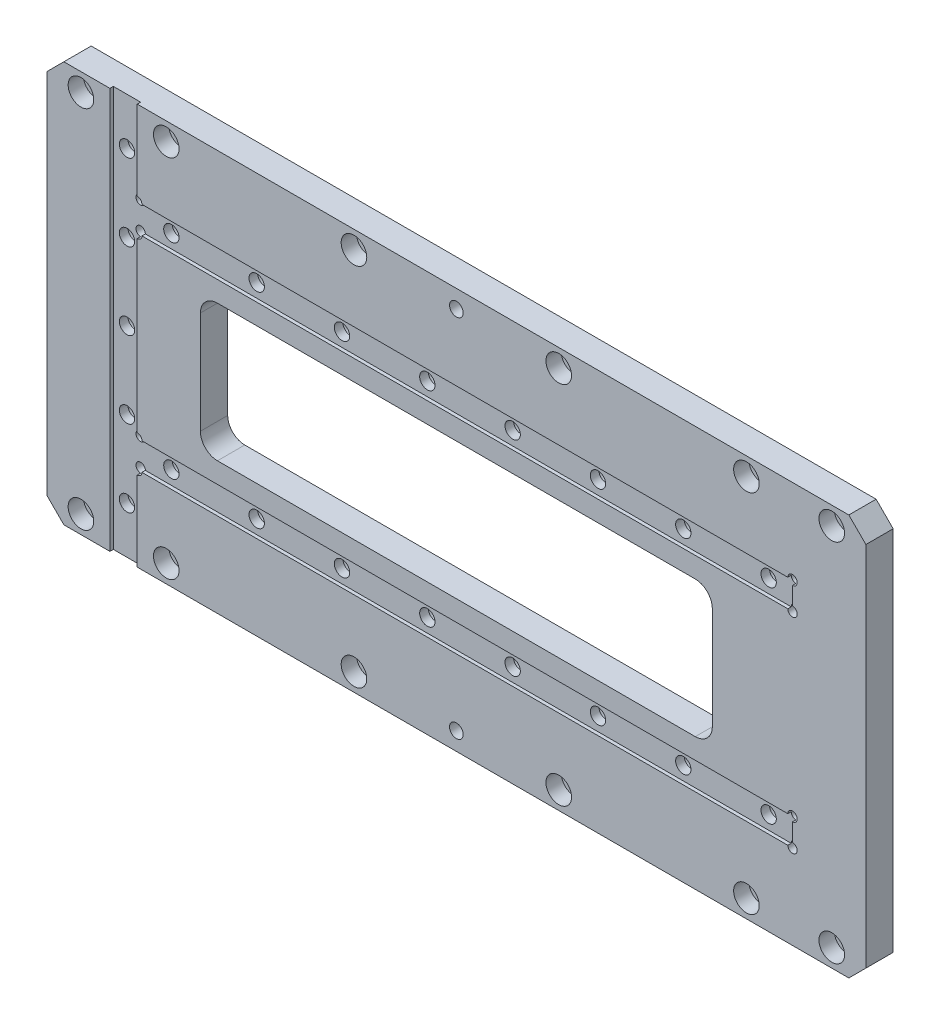
SolidWorks part; units mm, degrees
material "6061 合金"
ref_plane "Front" through (0, 0, 0) normal (0, 0, 1) x (1, 0, 0)
ref_plane "Top" through (0, 0, 0) normal (0, 1, 0) x (1, 0, 0)
ref_plane "Right" through (0, 0, 0) normal (1, 0, 0) x (0, 0, -1)
sketch "草图1" plane through (0, 0, 0) normal (0, 0, 1) x (1, 0, 0)
  line L2 (-240, -117.5) -> (-240, 117.5)
  line L3 (-240, 117.5) -> (240, 117.5)
  line L4 (240, -117.5) -> (240, 117.5)
  line L5 (-240, -117.5) -> (240, 117.5) construction
  line L6 (-240, 117.5) -> (240, -117.5) construction
  line L15 (-240, -117.5) -> (240, -117.5)
  dimension "D1" = 235
  dimension "D2" = 480
extrude "凸台-拉伸1" add sketch "草图1" along normal blind 16
hole_wizard "打孔尺寸(%根据)内六角圆柱头螺钉的类型1" positions "草图10" profile "草图11" counterbore size "M8" standard "GB" end condition through all
sketch "草图10" plane through (0, 0, 16) normal (0, 0, 1) x (1, 0, 0)
  line L8 (-220, 107) -> (220, 107) construction
  line L9 (-220, 107) -> (-220, -107) construction
  line L10 (-220, -107) -> (220, -107) construction
  line L11 (220, 107) -> (220, -107) construction
  line L12 (0, 117.5) -> (0, -117.2465) construction
  line L13 (-240, 117.5) -> (240, 117.5) construction
  line L14 (-240, 0) -> (240, 0) construction
  line L15 (-240, -117.5) -> (-240, 117.5) construction
  line L16 (240, -117.5) -> (240, 117.5) construction
  line L17 (-170, 107) -> (-170, -107) construction
  line L18 (-60, 107) -> (-60, -107) construction
  line L19 (60, 107) -> (60, -107) construction
  line L20 (170, 107) -> (170, -107) construction
  point P316 (-220, 107)
  point P317 (220, -107)
  point P420 (-220, -107)
  point P421 (220, 107)
  point P437 (-170, 107)
  point P438 (-170, -107)
  point P439 (-60, 107)
  point P440 (-60, -107)
  point P442 (60, 107)
  point P443 (60, -107)
  point P444 (170, 107)
  point P445 (170, -107)
  dimension "D1" = 214
  dimension "D2" = 440
  dimension "D3" = 120
  dimension "D4" = 340
sketch "草图11" plane through (-220, 107, 16) normal (1, 0, 0) x (0, -1, 0)
  line L0 (0, 0) -> (0, 16)
  line L1 (0, 16) -> (4.5, 16)
  line L3 (4.5, 16) -> (4.5, 9)
  line L4 (4.5, 9) -> (7.5, 9)
  line L5 (7.5, 9) -> (7.5, 0)
  line L7 (7.5, 0) -> (0, 0)
  line L11 (0, -6.35) -> (0, 107.95) construction
  dimension "通孔孔直径" = 9
  dimension "通孔孔深度" = 16
  dimension "柱形沉头孔直径" = 15
  dimension "柱形沉头孔深度" = 9
chamfer "倒角1" distance 10 angle 45 4 edges at (240, 117.5, 8) (240, -117.5, 8) (-240, -117.5, 8) (-240, 117.5, 8)
hole_wizard "大小mm 暗销孔1" positions "草图12" profile "草图13" hole size "Ø8.0" standard "GB" end condition through all
sketch "草图12" plane through (0, 0, 16) normal (0, 0, 1) x (1, 0, 0)
  line L1 (-60, 107) -> (60, 107) construction
  line L2 (-60, -107) -> (60, -107) construction
  point P12 (0, 107)
  point P14 (0, -107)
sketch "草图13" plane through (0, -107, 16) normal (1, 0, 0) x (0, -1, 0)
  line L0 (0, 0) -> (0, 16)
  line L1 (0, 16) -> (4, 16)
  line L2 (4, 16) -> (4, 0)
  line L5 (4, 0) -> (0, 0)
  line L11 (0, -6.35) -> (0, 107.95) construction
  dimension "通孔孔直径" = 8
  dimension "通孔孔深度" = 16
sketch "草图16" plane through (0, 0, 16) normal (0, 0, 1) x (1, 0, 0)
  line L0 (-240, 0) -> (240, 0) construction
  line L1 (-240, -107.5) -> (-240, 107.5) construction
  line L2 (240, -107.5) -> (240, 107.5) construction
  line L3 (-195, 117.5) -> (-195, -117.5) construction
  line L4 (-230, 117.5) -> (230, 117.5) construction
  line L5 (0, 117.5) -> (0, -117.5) construction
  line L6 (-230, -117.5) -> (230, -117.5) construction
  line L8 (-203, -117.5) -> (-187, -117.5)
  line L9 (-203, -117.5) -> (-203, 117.5)
  line L10 (-203, 117.5) -> (-187, 117.5)
  line L11 (-187, -117.5) -> (-187, 117.5)
  line L12 (-195, 117.5) -> (-195, -117.5) construction
  line L13 (-203, 0) -> (-187, 0) construction
  point P14 (-195, 0)
  dimension "D1" = 16
  dimension "D2" = 195
extrude "切除-拉伸1" cut sketch "草图16" against normal blind 2
sketch "草图17" plane through (0, 0, 16) normal (0, 0, 1) x (1, 0, 0)
  line L1 (-240, -107.5) -> (-240, 107.5) construction
  line L2 (-240, 0) -> (240, 0) construction
  line L3 (-203, 60) -> (-240, 60) construction
  line L4 (-203, 117.5) -> (-203, -117.5) construction
  line L5 (-240, -47.5) -> (-203, -47.5) construction
  line L6 (-203, -68) -> (-203, -52)
  line L7 (197, 68) -> (-203, 68)
  line L8 (197, 68) -> (197, 52)
  line L9 (197, 52) -> (-203, 52)
  line L10 (-203, 68) -> (-203, 52)
  line L11 (197, -52) -> (-203, -52)
  line L12 (197, -68) -> (197, -52)
  line L13 (197, -68) -> (-203, -68)
  line L14 (240, -107.5) -> (240, 107.5) construction
  dimension "D2" = 16
  dimension "D3" = 400
  dimension "D5" = 120
extrude "切除-拉伸2" cut sketch "草图17" against normal blind 2
sketch "草图18" plane through (0, 0, 16) normal (0, 0, 1) x (1, 0, 0)
  line L0 (-187, 52) -> (197, 52) construction
  line L1 (-150, -40) -> (150, -40)
  line L2 (-150, -40) -> (-150, 40)
  line L3 (-150, 40) -> (150, 40)
  line L4 (150, -40) -> (150, 40)
  line L5 (0, 40) -> (0, -40) construction
  point P0 (0, 0)
  dimension "D1" = 80
  dimension "D2" = 300
  dimension "D3" = 12
extrude "切除-拉伸3" cut sketch "草图18" against normal through all
fillet "圆角1" radius 10 4 edges at (-150, -40, 8) (-150, 40, 8) (150, -40, 8) (150, 40, 8)
hole_wizard "打孔尺寸(%根据)内六角圆柱头螺钉的类型3" positions "草图19" profile "草图20" counterbore size "M8" standard "GB" end condition through all
sketch "草图19" plane through (0, 0, 0) normal (0, 0, -1) x (-1, 0, 0)
  line L0 (195, 117.5) -> (195, -117.5) construction
  line L1 (230, 117.5) -> (-230, 117.5) construction
  line L4 (187, 68) -> (187, 117.5) construction
  line L5 (203, 117.5) -> (203, -117.5) construction
  line L6 (187, 92.75) -> (203, 92.75) construction
  line L7 (195, 92.75) -> (195, 93.75) construction
  line L8 (195, 92.75) -> (195, 145.0943) construction
  line L9 (195, -92.75) -> (195, -93.75) construction
  line L10 (187, -92.75) -> (203, -92.75) construction
  line L11 (230, -117.5) -> (-230, -117.5) construction
  line L12 (-150, 0) -> (309.2461, 0) construction
  line L13 (-150, -30) -> (-150, 30) construction
  point P25 (195, 45)
  point P27 (195, 90)
  point P36 (195, -90)
  point P37 (195, -45)
  point P39 (195, 0)
  dimension "D1" = 45
  dimension "D2" = 27.5
  dimension "D4" = 45
  dimension "D5" = 45
  dimension "D6" = 45
sketch "草图20" plane through (-195, 0, 0) normal (1, 0, 0) x (0, 1, 0)
  line L0 (0, 0) -> (0, 16)
  line L1 (0, 16) -> (4.5, 16)
  line L3 (4.5, 16) -> (4.5, 9)
  line L4 (4.5, 9) -> (7.5, 9)
  line L5 (7.5, 9) -> (7.5, 0)
  line L7 (7.5, 0) -> (0, 0)
  line L11 (0, -6.35) -> (0, 107.95) construction
  dimension "通孔孔直径" = 9
  dimension "通孔孔深度" = 16
  dimension "柱形沉头孔直径" = 15
  dimension "柱形沉头孔深度" = 9
hole_wizard "打孔尺寸(%根据)内六角圆柱头螺钉的类型3" positions "草图21" profile "草图22" counterbore size "M8" standard "GB" end condition through all
sketch "草图21" plane through (0, 0, 0) normal (0, 0, -1) x (-1, 0, 0)
  line L0 (240, 0) -> (-240, 0) construction
  line L1 (240, -107.5) -> (240, 107.5) construction
  line L2 (-240, -107.5) -> (-240, 107.5) construction
  line L3 (-197, 60) -> (203, 60) construction
  line L4 (-197, 52) -> (-197, 68) construction
  line L5 (203, 117.5) -> (203, -117.5) construction
  line L6 (-197, -60) -> (203, -60) construction
  line L7 (-197, -68) -> (-197, -52) construction
  line L8 (169, 60) -> (169, -60) construction
  point P16 (169, 60)
  point P17 (169, -60)
  dimension "D1" = 34
sketch "草图22" plane through (-169, -60, 0) normal (1, 0, 0) x (0, 1, 0)
  line L0 (0, 0) -> (0, 16)
  line L1 (0, 16) -> (4.5, 16)
  line L3 (4.5, 16) -> (4.5, 9)
  line L4 (4.5, 9) -> (7.5, 9)
  line L5 (7.5, 9) -> (7.5, 0)
  line L7 (7.5, 0) -> (0, 0)
  line L11 (0, -6.35) -> (0, 107.95) construction
  dimension "通孔孔直径" = 9
  dimension "通孔孔深度" = 16
  dimension "柱形沉头孔直径" = 15
  dimension "柱形沉头孔深度" = 9
pattern_linear "阵列(线性)1" count 8 spacing 50 along (1, 0, 0) of "打孔尺寸(%根据)内六角圆柱头螺钉的类型3"
hole_wizard "Ø5.5 (5.5) 直径孔1" positions "草图23" profile "草图24" hole size "Ø5.5" standard "GB" end condition through all
sketch "草图23" plane through (0, 0, 16) normal (0, 0, 1) x (1, 0, 0)
  line L0 (-187, -68) -> (197, -68) construction
  line L1 (197, 52) -> (197, 68) construction
  line L2 (197, 52) -> (197, 68) construction
  line L3 (-187, -52) -> (-187, 52) construction
  line L4 (197, -52) -> (-187, -52) construction
  point P0 (197, -68)
  point P4 (197, -52)
  point P7 (197, 52)
  point P10 (197, 68)
  point P16 (-187, 68)
  point P19 (-187, 52)
  point P22 (-187, -68)
  point P25 (-187, -52)
sketch "草图24" plane through (197, -68, 16) normal (1, 0, 0) x (0, -1, 0)
  line L0 (0, 0) -> (0, 16)
  line L1 (0, 16) -> (2.75, 16)
  line L2 (2.75, 16) -> (2.75, 0)
  line L5 (2.75, 0) -> (0, 0)
  line L11 (0, -6.35) -> (0, 107.95) construction
  dimension "通孔孔直径" = 5.5
  dimension "通孔孔深度" = 16
